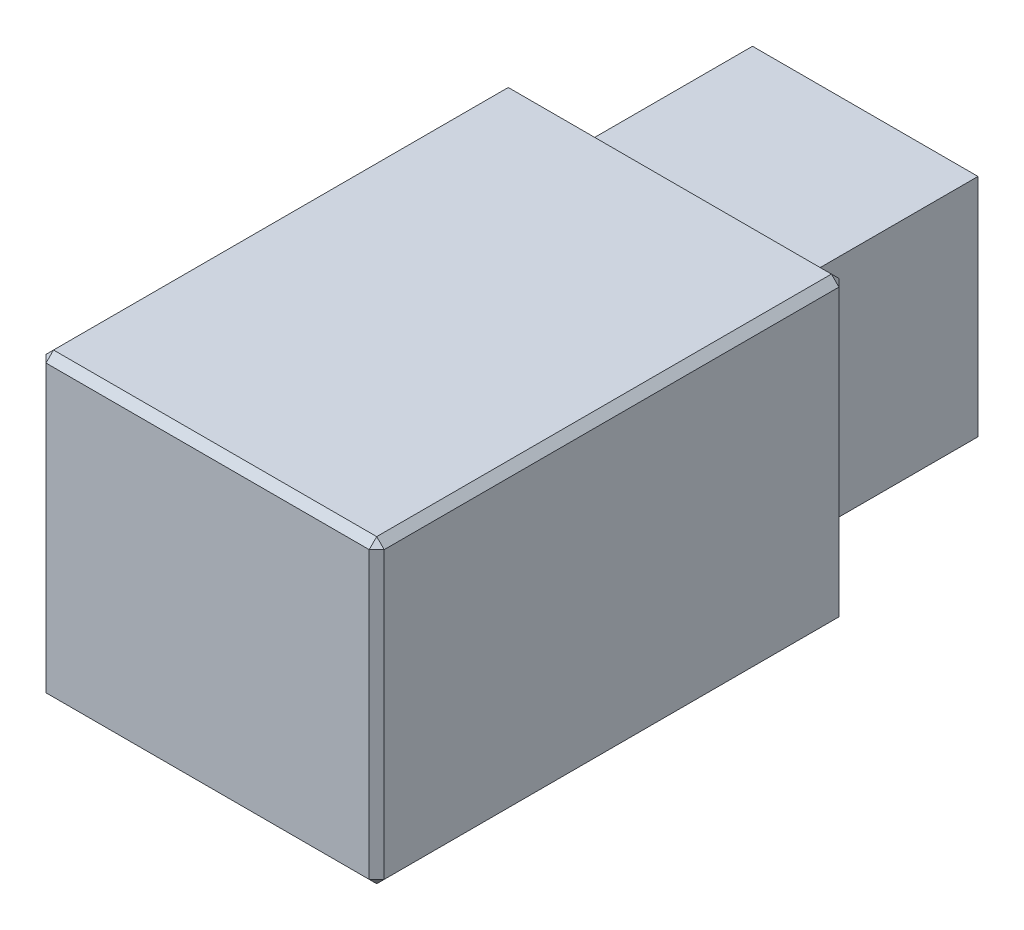
from build123d import *

# Parameters (mm, degrees)
SKETCH_1_W          = 60
SKETCH_1_H          = 60
EXTRUDE_227_DEPTH   = 50
SKETCH_2_W          = 90
SKETCH_2_H          = 80
EXTRUDE_1_DEPTH     = 125
CHAMFER_1_SIZE      = 2
SKETCH_3_R          = 6
CUT_EXTRUDE_1_DEPTH = 80


with BuildPart() as part:
    # 草图1 → Extrude 227 (new body)
    with BuildSketch(Plane.XY):
        with Locations((30, 30)):
            Rectangle(SKETCH_1_W, SKETCH_1_H)
    extrude(amount=EXTRUDE_227_DEPTH)

    # 草图2 → 凸台-拉伸1 (add)
    with BuildSketch(Plane.XY.offset(50)):
        with Locations((30, 30)):
            Rectangle(SKETCH_2_W, SKETCH_2_H)
    extrude(amount=EXTRUDE_1_DEPTH)

    # 倒角1
    chamfer_1_edges = [part.edges().sort_by_distance(p)[0] for p in [
        (-15, 70, 112.5),
        (75, 70, 112.5),
        (30, 70, 50),
        (30, 70, 175),
        (-15, -10, 112.5),
        (-15, 30, 50),
        (-15, 30, 175),
        (75, -10, 112.5),
        (75, 30, 50),
        (75, 30, 175),
        (30, -10, 50),
        (0, 30, 50),
        (30, 60, 50),
        (60, 30, 50),
        (30, 0, 50),
        (30, -10, 175),
    ]]
    chamfer(chamfer_1_edges, length=CHAMFER_1_SIZE)

    # 草图3 → 切除-拉伸1 (cut)
    with BuildSketch(Plane(origin=(0, 0, 0), x_dir=(-1, 0, 0), z_dir=(0, 0, -1))):
        with Locations((-30, 30)):
            Circle(SKETCH_3_R)
    extrude(amount=-CUT_EXTRUDE_1_DEPTH, mode=Mode.SUBTRACT)


solid = part.part
